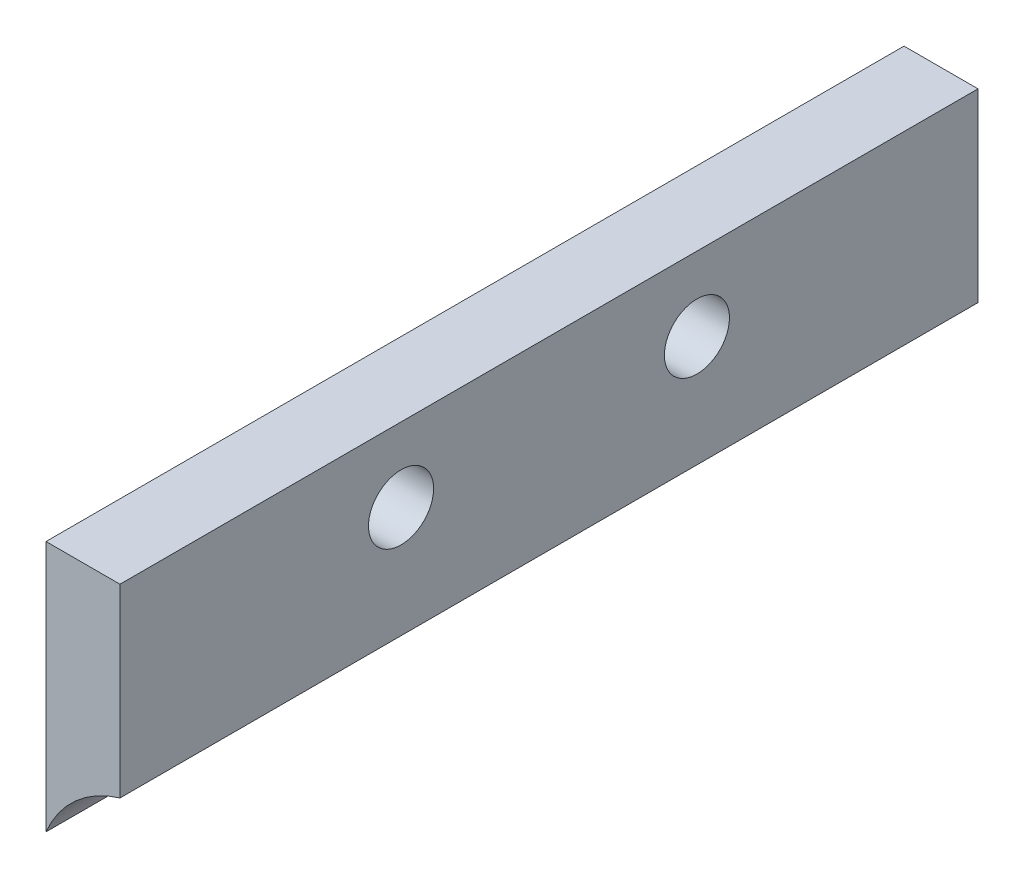
SolidWorks part; units mm, degrees
ref_plane "前视基准面" through (0, 0, 0) normal (0, 0, 1) x (1, 0, 0)
ref_plane "上视基准面" through (0, 0, 0) normal (0, 1, 0) x (1, 0, 0)
ref_plane "右视基准面" through (0, 0, 0) normal (1, 0, 0) x (0, 0, -1)
sketch "草图1" plane through (0, 0, 0) normal (0, 0, 1) x (1, 0, 0)
  line L1 (-3.0117, 4.5415) -> (1.9883, 4.5415)
  line L2 (-3.0117, 4.5415) -> (-3.0117, -12.4585)
  line L4 (1.9883, 4.5415) -> (1.9883, -7.9752)
  arc A0 (1.9883, -7.9752) -> (-3.0117, -12.4585) centre (4.1883, -15.4585) ccw
  dimension "D5" = 15.6
  dimension "D1" = 5
extrude "凸台-拉伸1" add sketch "草图1" along normal blind 58
sketch "草图2" plane through (1.9883, 0, 0) normal (1, 0, 0) x (0, 0, -1)
  line L0 (-58, 4.5415) -> (0, 4.5415) construction
  line L1 (0, -7.9752) -> (0, 4.5415) construction
  line L2 (-58, -7.9752) -> (-58, 4.5415) construction
  circle A0 centre (-19, -0.4585) radius 2.2
  circle A1 centre (-39, -0.4585) radius 2.2
  dimension "D5" = 4.4
  dimension "D6" = 4.4
  dimension "D1" = 5
  dimension "D2" = 19
  dimension "D3" = 5
  dimension "D4" = 19
extrude "切除-拉伸1" cut sketch "草图2" against normal blind 10
